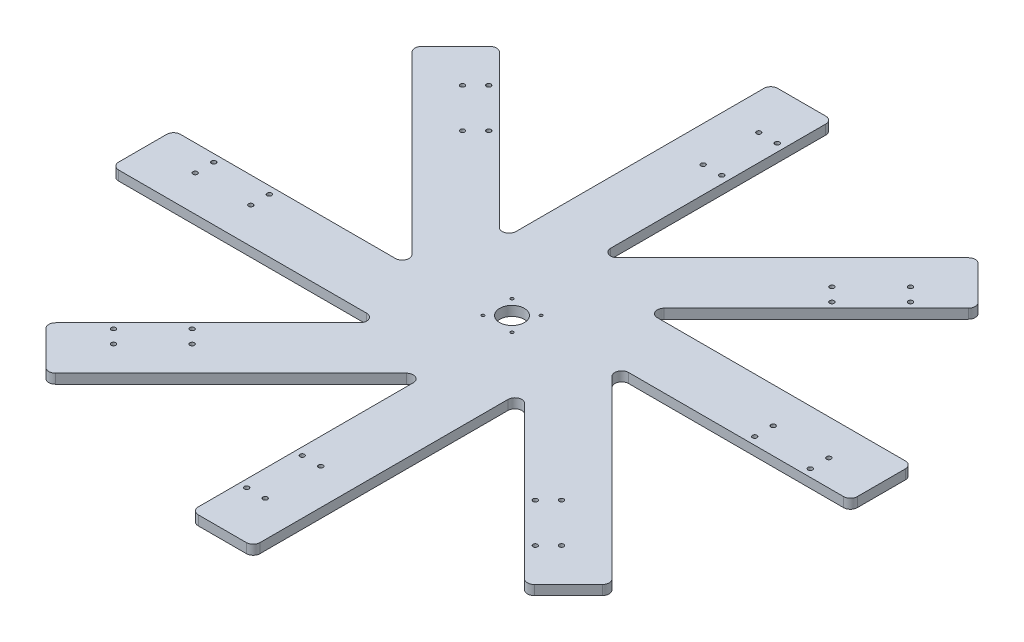
from build123d import *

# Parameters (mm, degrees)
SKETCH_3_R               = 50
SKETCH_3_R_2             = 18
EXTRUDE_4_DEPTH          = 7
SKETCH_4_W               = 462
SKETCH_4_H               = 90
EXTRUDE_5_DEPTH          = 7
SKETCH_5_R               = 3.3
CUT_EXTRUDE_7_DEPTH      = 30
FILLET_2_R               = 10
PATTERN_CIRCULAR_1_COUNT = 8
FILLET_1_R               = 10
FILLET_3_R               = 10
SKETCH_7_R               = 30
SKETCH_7_R_2             = 18
EXTRUDE_6_DEPTH          = 15
SKETCH_8_R               = 2.75
CUT_EXTRUDE_3_DEPTH      = 50
CUT_EXTRUDE_START        = -29
SKETCH_9_R               = 5
CUT_EXTRUDE_4_DEPTH      = 103
PATTERN_CIRCULAR_2_COUNT = 4
SKETCH_11_R              = 87.380372297
CUT_EXTRUDE_5_DEPTH      = 51
SKETCH_12_R              = 2.2
CUT_EXTRUDE_6_DEPTH      = 51
PATTERN_CIRCULAR_3_COUNT = 4


with BuildPart() as part:
    # 草图3 → 凸台-拉伸4 (new, symmetric)
    with BuildSketch(Plane(origin=(0, 0, 0), x_dir=(1, 0, 0), z_dir=(0, 1, 0))):
        with Locations(Location((0, 0, 0), (0, 0, 270))):
            Circle(SKETCH_3_R)
        with Locations(Location((0, 0, 0), (0, 0, 270))):
            Circle(SKETCH_3_R_2, mode=Mode.SUBTRACT)
    extrude(amount=EXTRUDE_4_DEPTH, both=True)

    # 草图4 → 凸台-拉伸5 (add, symmetric)
    with BuildSketch(Plane(origin=(0, 0, 0), x_dir=(1, 0, 0), z_dir=(0, 1, 0))):
        with Locations((249, 58)):
            Rectangle(SKETCH_4_W, SKETCH_4_H)
    extrude_5 = extrude(amount=EXTRUDE_5_DEPTH, both=True)

    # 草图5 → 切除-拉伸7 (cut)
    with BuildSketch(Plane(origin=(0, 7, 0), x_dir=(1, 0, 0), z_dir=(0, 1, 0))):
        with Locations(Location((329.5, 51, 0), (0, 0, 270))):
            Circle(SKETCH_5_R)
        with Locations(Location((329.5, 24, 0), (0, 0, 270))):
            Circle(SKETCH_5_R)
        with Locations(Location((410.5, 51, 0), (0, 0, 270))):
            Circle(SKETCH_5_R)
        with Locations(Location((410.5, 24, 0), (0, 0, 270))):
            Circle(SKETCH_5_R)
    cut_extrude_7 = extrude(amount=-CUT_EXTRUDE_7_DEPTH, mode=Mode.SUBTRACT)

    # 圆角2
    fillet_2_edges = [part.edges().sort_by_distance(p)[0] for p in [
        (480, 0, -13),
        (480, 0, -103),
    ]]
    fillet(fillet_2_edges, radius=FILLET_2_R)

    # 阵列(圆周)1: 凸台-拉伸5, 切除-拉伸7 ×8 about axis
    pattern_circular_1_axis = Axis((0, 0, 0), (0, 1, 0))
    add([extrude_5.rotate(pattern_circular_1_axis, i * 360 / PATTERN_CIRCULAR_1_COUNT) for i in range(1, PATTERN_CIRCULAR_1_COUNT)])
    add([cut_extrude_7.rotate(pattern_circular_1_axis, i * 360 / PATTERN_CIRCULAR_1_COUNT) for i in range(1, PATTERN_CIRCULAR_1_COUNT)], mode=Mode.SUBTRACT)

    # 圆角1
    fillet_1_edges = [part.edges().sort_by_distance(p)[0] for p in [
        (-13, 0, -132.663996924),
        (84.615223689, 0, -103),
        (132.663996924, 0, -13),
        (103, 0, 84.615223689),
        (13, 0, 132.663996924),
        (-84.615223689, 0, 103),
        (-132.663996924, 0, 13),
        (-103, 0, -84.615223689),
    ]]
    fillet(fillet_1_edges, radius=FILLET_1_R)

    # 圆角3
    fillet_3_edges = [part.edges().sort_by_distance(p)[0] for p in [
        (-13, 0, -480),
        (266.579256507, 0, -412.243253432),
        (330.218866814, 0, -348.603643125),
        (412.243253432, 0, 266.579256507),
        (348.603643125, 0, 330.218866814),
        (103, 0, 480),
        (13, 0, 480),
        (-266.579256507, 0, 412.243253432),
        (-330.218866814, 0, 348.603643125),
        (-480, 0, 103),
        (-480, 0, 13),
        (-412.243253432, 0, -266.579256507),
        (-348.603643125, 0, -330.218866814),
        (-103, 0, -480),
    ]]
    fillet(fillet_3_edges, radius=FILLET_3_R)

    # 草图7 → 凸台-拉伸6 (add)
    with BuildSketch(Plane(origin=(0, 7, 0), x_dir=(1, 0, 0), z_dir=(0, 1, 0))):
        with Locations(Location((0, 0, 0), (0, 0, 270))):
            Circle(SKETCH_7_R)
        with Locations(Location((0, 0, 0), (0, 0, 270))):
            Circle(SKETCH_7_R_2, mode=Mode.SUBTRACT)
    extrude(amount=EXTRUDE_6_DEPTH)

    # 草图8 → 切除-拉伸3 (cut)
    with BuildSketch(Plane(origin=(0, 0, 0), x_dir=(0, 0, -1), z_dir=(1, 0, 0))):
        with Locations((0, 15)):
            Circle(SKETCH_8_R)
    cut_extrude_3 = extrude(amount=-CUT_EXTRUDE_3_DEPTH, mode=Mode.SUBTRACT)

    # 草图9 → 切除-拉伸4 (cut)
    with BuildSketch(Plane(origin=(0, 0, 0), x_dir=(0, 0, -1), z_dir=(1, 0, 0)).offset(CUT_EXTRUDE_START)):
        with Locations((0, 15)):
            Circle(SKETCH_9_R)
    cut_extrude_4 = extrude(amount=-CUT_EXTRUDE_4_DEPTH, mode=Mode.SUBTRACT)

    # 阵列(圆周)2: 切除-拉伸3, 切除-拉伸4 ×4 about axis
    pattern_circular_2_axis = Axis((0, 0, 0), (0, 1, 0))
    add([cut_extrude_3.rotate(pattern_circular_2_axis, i * 360 / PATTERN_CIRCULAR_2_COUNT) for i in range(1, PATTERN_CIRCULAR_2_COUNT)], mode=Mode.SUBTRACT)
    add([cut_extrude_4.rotate(pattern_circular_2_axis, i * 360 / PATTERN_CIRCULAR_2_COUNT) for i in range(1, PATTERN_CIRCULAR_2_COUNT)], mode=Mode.SUBTRACT)

    # 草图11 → 切除-拉伸5 (cut)
    with BuildSketch(Plane(origin=(0, 7, 0), x_dir=(1, 0, 0), z_dir=(0, 1, 0))):
        Circle(SKETCH_11_R)
    extrude(amount=CUT_EXTRUDE_5_DEPTH, mode=Mode.SUBTRACT)

    # 草图12 → 切除-拉伸6 (cut)
    with BuildSketch(Plane(origin=(0, 7, 0), x_dir=(1, 0, 0), z_dir=(0, 1, 0))):
        with Locations(Location((21.213203436, 21.213203436, 0), (0, 0, 270))):
            Circle(SKETCH_12_R)
    cut_extrude_6 = extrude(amount=-CUT_EXTRUDE_6_DEPTH, mode=Mode.SUBTRACT)

    # 阵列(圆周)3: 切除-拉伸6 ×4 about axis
    pattern_circular_3_axis = Axis((0, 0, 0), (0, 1, 0))
    for i in range(1, PATTERN_CIRCULAR_3_COUNT):
        add(cut_extrude_6.rotate(pattern_circular_3_axis, i * 360 / PATTERN_CIRCULAR_3_COUNT), mode=Mode.SUBTRACT)


solid = part.part
